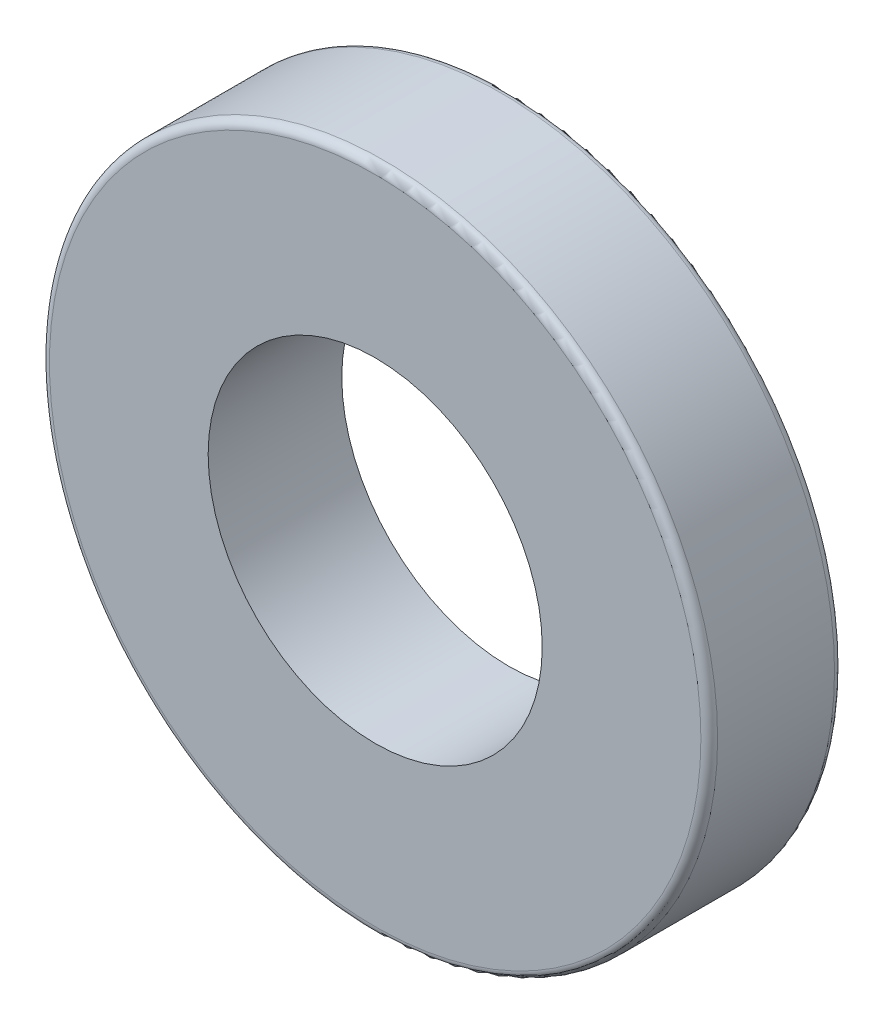
from build123d import *

# Parameters (mm, degrees)
SKETCH_1_R      = 20
SKETCH_1_R_2    = 10
EXTRUDE_1_DEPTH = 4
FILLET_1_R      = 0.5


with BuildPart() as part:
    # 草图1 → 凸台-拉伸1 (new, symmetric)
    with BuildSketch(Plane.XY):
        Circle(SKETCH_1_R)
        Circle(SKETCH_1_R_2, mode=Mode.SUBTRACT)
    extrude(amount=EXTRUDE_1_DEPTH, both=True)

    # 圆角1
    fillet_1_edges = [part.edges().sort_by_distance(p)[0] for p in [
        (-20, 0, -4),
        (-20, 0, 4),
    ]]
    fillet(fillet_1_edges, radius=FILLET_1_R)


solid = part.part
